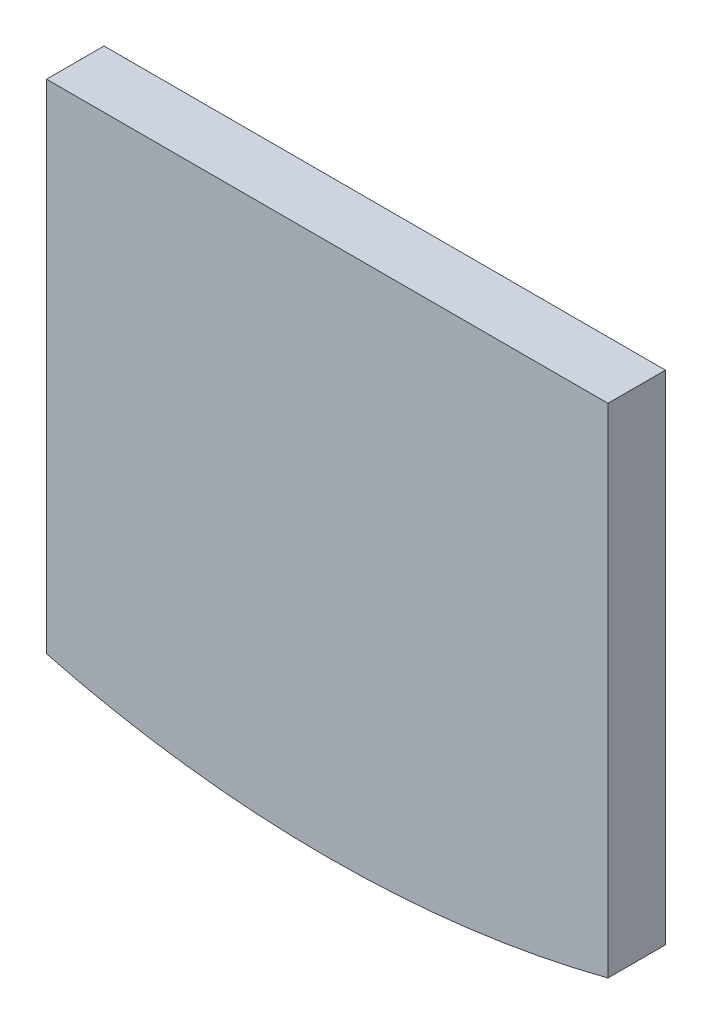
SolidWorks part; units mm, degrees
material "普通碳钢"
ref_plane "Front Plane" through (0, 0, 0) normal (0, 0, 1) x (1, 0, 0)
ref_plane "Top Plane" through (0, 0, 0) normal (0, 1, 0) x (1, 0, 0)
ref_plane "Right Plane" through (0, 0, 0) normal (1, 0, 0) x (0, 0, -1)
sketch "Sketch1" plane through (0, 0, 0) normal (0, 0, 1) x (1, 0, 0)
  line L0 (0, 419.1) -> (0, -362.6741) construction
  line L1 (-127, 152.4) -> (127, 152.4)
  line L2 (-127, 152.4) -> (-127, -88.9) construction
  line L3 (-127, -88.9) -> (127, -88.9) construction
  line L4 (127, 152.4) -> (127, -88.9) construction
  line L5 (-127, 152.4) -> (-127, -72.7689)
  line L6 (127, 152.4) -> (127, -72.7689)
  arc A0 (-127, -72.7689) -> (127, -72.7689) centre (0, 419.1) ccw
  dimension "D1" = 254
  dimension "D5" = 1016
  dimension "D2" = 241.3
  dimension "D3" = 127
  dimension "D4" = 152.4
extrude "Boss-Extrude1" add sketch "Sketch1" along normal mid plane 26
